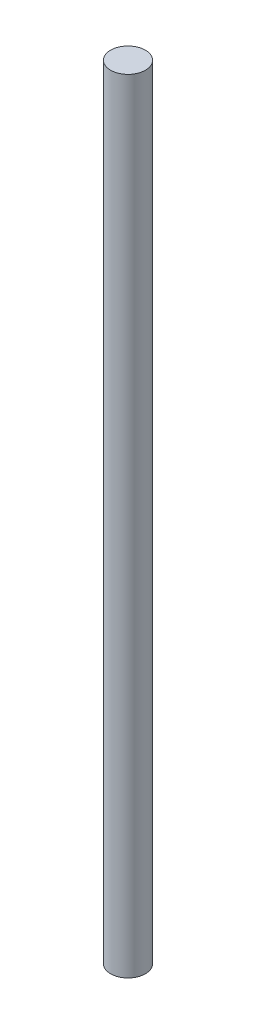
SolidWorks part; units mm, degrees
ref_plane "Front" through (0, 0, 0) normal (0, 0, 1) x (1, 0, 0)
ref_plane "Top" through (0, 0, 0) normal (0, 1, 0) x (1, 0, 0)
ref_plane "Right" through (0, 0, 0) normal (1, 0, 0) x (0, 0, -1)
sketch "草图1" plane through (0, 0, 0) normal (0, 1, 0) x (1, 0, 0)
  circle A0 centre (0, 0) radius 4
  dimension "D1" = 8
extrude "凸台-拉伸1" add sketch "草图1" along normal blind 180
